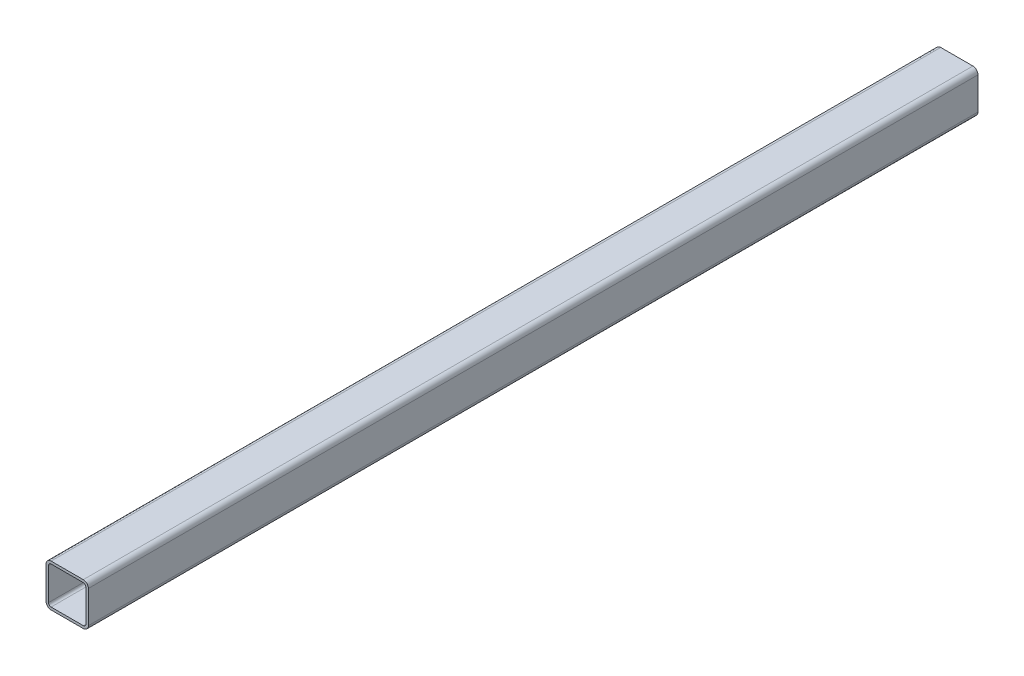
SolidWorks part; units mm, degrees
material "Q235B"
ref_plane "前视基准面" through (0, 0, 0) normal (0, 0, 1) x (1, 0, 0)
ref_plane "上视基准面" through (0, 0, 0) normal (0, 1, 0) x (1, 0, 0)
ref_plane "右视基准面" through (0, 0, 0) normal (1, 0, 0) x (0, 0, -1)
other "Configuration Table"
sketch "草图1" plane through (0, 0, 0) normal (1, 0, 0) x (0, 0, -1)
  line L0 (-525, 0) -> (525, 0)
other "Gb／6728-1986方形空心型钢 050 X 50 X 3(1)"
ref_plane "基准面1" through (0, 0, 525) normal (0, 0, -1) x (0, 1, 0)
sketch "Sketch1" plane through (0, 0, 525) normal (0, 0, -1) x (0, 1, 0)
  line L0 (-19, -22) -> (19, -22)
  line L1 (-22, -19) -> (-22, 19)
  line L2 (19, 22) -> (-19, 22)
  line L3 (22, 19) -> (22, -19)
  line L4 (-19, -25) -> (19, -25)
  line L5 (-25, -19) -> (-25, 19)
  line L6 (19, 25) -> (-19, 25)
  line L7 (25, 19) -> (25, -19)
  arc A0 (25, 19) -> (19, 25) centre (19, 19) ccw
  arc A1 (19, -25) -> (25, -19) centre (19, -19) ccw
  arc A2 (-25, -19) -> (-19, -25) centre (-19, -19) ccw
  arc A3 (-19, 25) -> (-25, 19) centre (-19, 19) ccw
  arc A4 (-19, 22) -> (-22, 19) centre (-19, 19) ccw
  arc A5 (22, 19) -> (19, 22) centre (19, 19) ccw
  arc A6 (19, -22) -> (22, -19) centre (19, -19) ccw
  arc A7 (-22, -19) -> (-19, -22) centre (-19, -19) ccw
  point P0 (-25, 0)
  point P1 (25, 0)
  point P2 (0, 25)
  point P3 (0, -25)
  point P4 (0, 0)
  point P5 (-25, -25)
  point P6 (25, -25)
  point P7 (25, 25)
  point P8 (-25, 25)
  point P33 (0, 0)
  dimension "D1" = 6
  dimension "Thickness" = 3
  dimension "V_leg" = 50
equation "\"D2@草图1\"=\"D1@草图1\"/2"
